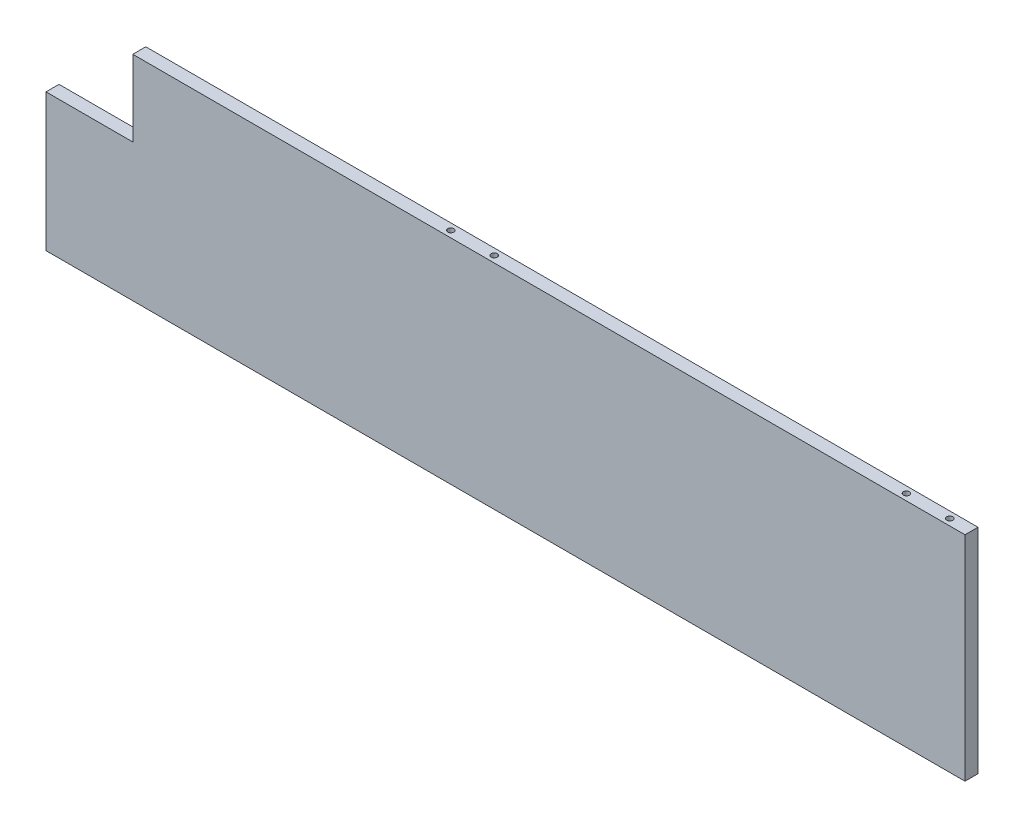
SolidWorks part; units mm, degrees
material "Q235"
ref_plane "Front Plane" through (0, 0, 0) normal (0, 0, 1) x (1, 0, 0)
ref_plane "Top Plane" through (0, 0, 0) normal (0, 1, 0) x (1, 0, 0)
ref_plane "Right Plane" through (0, 0, 0) normal (1, 0, 0) x (0, 0, -1)
sketch "Sketch1" plane through (0, 0, 0) normal (0, 0, 1) x (1, 0, 0)
  line L0 (0, 317) -> (200, 317)
  line L1 (0, 0) -> (2118, 0)
  line L2 (0, 0) -> (0, 317)
  line L3 (200, 492) -> (2118, 492)
  line L4 (2118, 0) -> (2118, 492)
  line L5 (200, 317) -> (200, 492)
  dimension "D1" = 2118
  dimension "D2" = 492
  dimension "D3" = 200
  dimension "D4" = 175
extrude "Boss-Extrude1" add sketch "Sketch1" along normal blind 30
hole_wizard "M16 Tapped Hole1" positions "3DSketch1" profile "Sketch2" tap size "M16" standard "GB"
sketch3d "3DSketch1"
  line L0 (2118, 492, 0) -> (200, 492, 0) construction
  line L1 (2118, 492, 30) -> (2118, 492, 0) construction
  point P0 (918, 492, 15)
  point P2 (1018, 492, 15)
  point P4 (2068, 492, 15)
  point P6 (1968, 492, 15)
  dimension "D1" = 50
  dimension "D2" = 15
  dimension "D3" = 100
  dimension "D4" = 1200
  dimension "D5" = 100
sketch "Sketch2" plane through (918, 492, 15) normal (1, 0, 0) x (0, 0, 1)
  line L0 (0, 0) -> (0, 49.206)
  line L1 (0, 49.206) -> (7, 45)
  line L2 (7, 45) -> (7, 0)
  line L5 (7, 0) -> (0, 0)
  line L10 (0, 49.206) -> (-7, 45) construction
  line L11 (0, -6.35) -> (0, 107.95) construction
  dimension "螺纹孔钻头直径" = 14
  dimension "螺纹孔钻头深度" = 45
  dimension "导头角度" = 118
cosmetic thread "Cosmetic thread 1" parameters "D1"=30, "D2"=16
cosmetic thread "Cosmetic thread 2" parameters "D1"=30, "D2"=16
cosmetic thread "Cosmetic thread 3" parameters "D1"=30, "D2"=16
cosmetic thread "Cosmetic thread 4" parameters "D1"=30, "D2"=16
